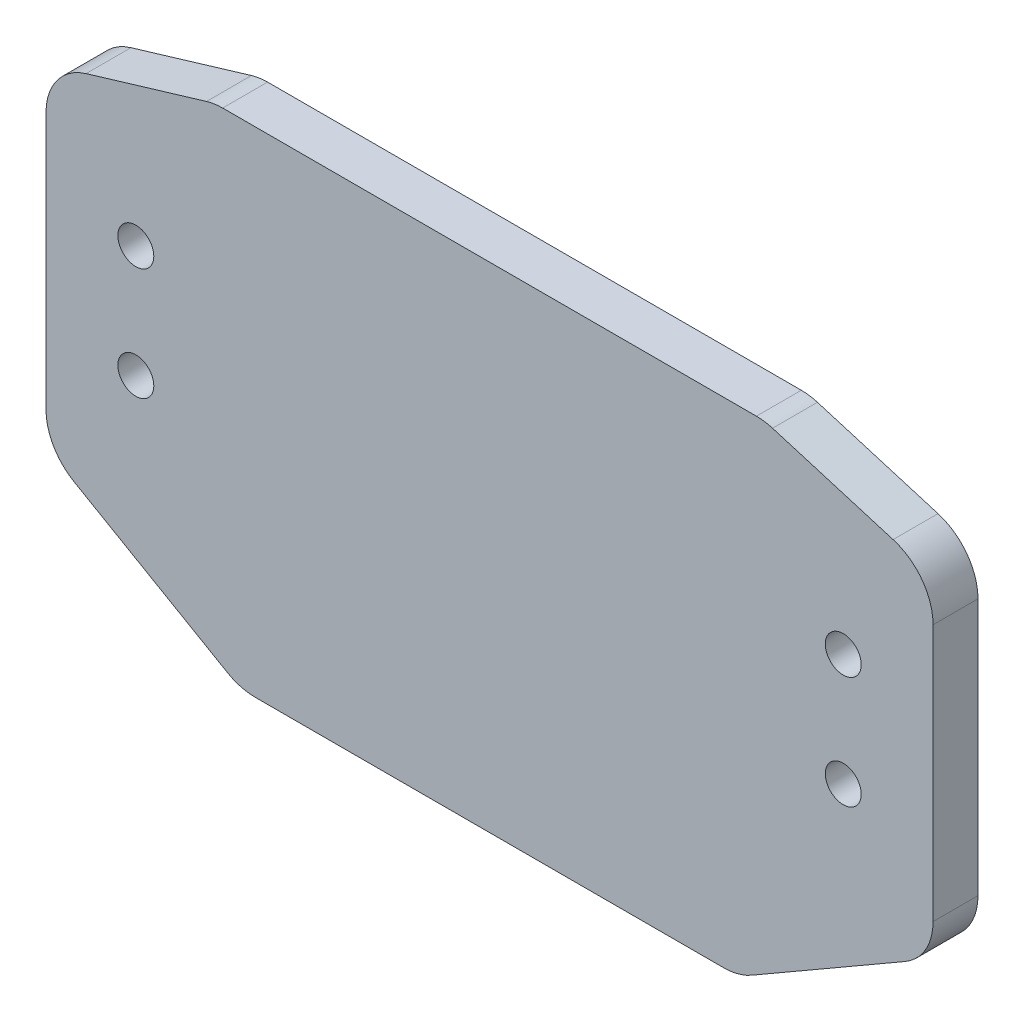
SolidWorks part; units mm, degrees
material "ABS PC"
ref_plane "Front Plane" through (0, 0, 0) normal (0, 0, 1) x (1, 0, 0)
ref_plane "Top Plane" through (0, 0, 0) normal (0, 1, 0) x (1, 0, 0)
ref_plane "Right Plane" through (0, 0, 0) normal (1, 0, 0) x (0, 0, -1)
sketch "Sketch1" plane through (0, 0, 0) normal (0, 0, 1) x (1, 0, 0)
  line L0 (0, 23.5) -> (0, -20.5) construction
  line L1 (-24.5, 23.5) -> (24.5, 23.5)
  line L2 (-39.5, 19) -> (-39.5, -10.5)
  line L3 (-22.1795, -20.5) -> (22.1795, -20.5)
  line L4 (39.5, 19) -> (39.5, -10.5)
  line L5 (-39.5, -10.5) -> (-22.1795, -20.5)
  line L6 (-39.5, 19) -> (-24.5, 23.5)
  line L7 (-31.5, 9) -> (-31.5, -1) construction
  line L8 (31.5, 9) -> (31.5, -1) construction
  line L9 (39.5, -10.5) -> (22.1795, -20.5)
  line L10 (39.5, 19) -> (24.5, 23.5)
  circle A0 centre (-31.5, 9) radius 1.6
  circle A1 centre (-31.5, -1) radius 1.6
  circle A2 centre (31.5, -1) radius 1.6
  circle A3 centre (31.5, 9) radius 1.6
  circle A4 centre (0, 0) radius 19.5 construction
  point P0 (0, 0)
  dimension "D1" = 79
  dimension "D4" = 3.2
  dimension "D7" = 39
  dimension "D2" = 10
  dimension "D3" = 8
  dimension "D5" = 1
  dimension "D6" = 44
  dimension "D8" = 14.5
  dimension "D9" = 10
  dimension "D10" = 49
  dimension "D11" = 120
  dimension "D12" = 10
extrude "Boss-Extrude1" add sketch "Sketch1" along normal blind 4
fillet "R5 Fillet 1" radius 5 8 edges at (-39.5, -10.5, 2) (-22.1795, -20.5, 2) (22.1795, -20.5, 2) (39.5, -10.5, 2) (39.5, 19, 2) (24.5, 23.5, 2) (-24.5, 23.5, 2) (-39.5, 19, 2)
